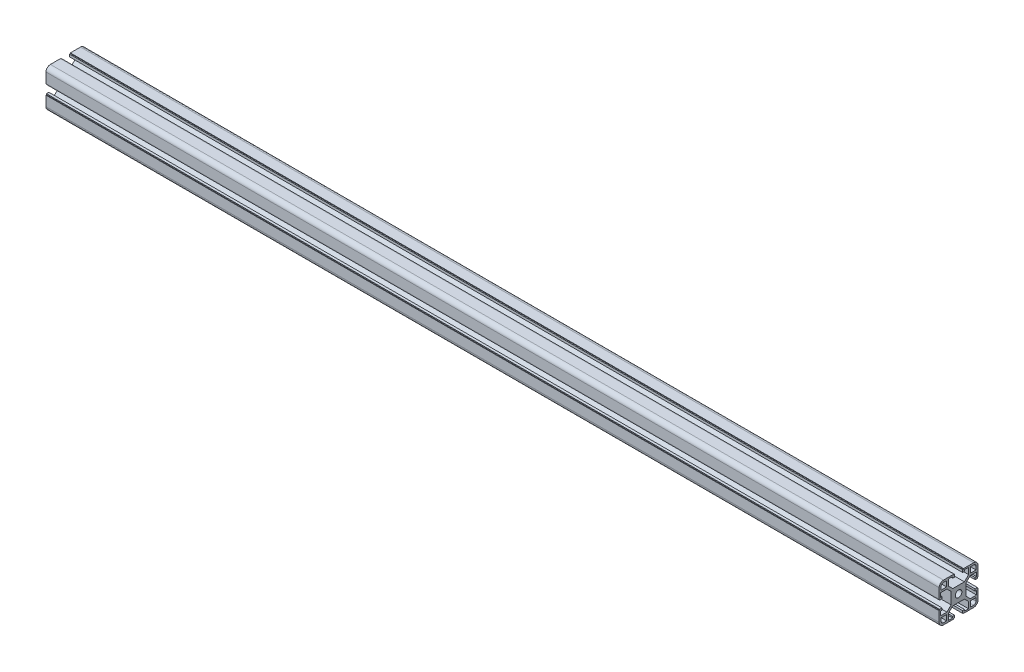
from build123d import *

# Parameters (mm, degrees)
SKETCH1_R                                = 3.4
ALUMINUM_PROFILE_40_X_40B_X_R4_5_1_DEPTH = 920


with BuildPart() as part:
    # Sketch1 → Aluminum profile 40 X 40B X R4.5(1) (new body)
    with BuildSketch(Plane.YZ):
        with BuildLine():
            Line((-5.1, 20), (-5.1, 19.5))
            Line((-5.1, 19.5), (-4.1, 19.5))
            Line((-4.1, 19.5), (-4.1, 17))
            Line((-4.1, 17), (-6.1, 17))
            Line((-6.1, 17), (-6.1, 18.5))
            Line((-6.1, 18.5), (-10.3, 18.5))
            Line((-10.3, 18.5), (-10.3, 12))
            Line((-10.3, 12), (-6, 7.7))
            Line((-6, 7.7), (6, 7.7))
            Line((6, 7.7), (10.3, 12))
            Line((10.3, 12), (10.3, 18.5))
            Line((10.3, 18.5), (6.1, 18.5))
            Line((6.1, 18.5), (6.1, 17))
            Line((6.1, 17), (4.1, 17))
            Line((4.1, 17), (4.1, 19.5))
            Line((4.1, 19.5), (5.1, 19.5))
            Line((5.1, 19.5), (5.1, 20))
            Line((5.1, 20), (15.5, 20))
            ThreePointArc((15.5, 20), (18.681980515, 18.681980515), (20, 15.5))
            Line((20, 15.5), (20, 5.1))
            Line((20, 5.1), (19.5, 5.1))
            Line((19.5, 5.1), (19.5, 4.1))
            Line((19.5, 4.1), (17, 4.1))
            Line((17, 4.1), (17, 6.1))
            Line((17, 6.1), (18.5, 6.1))
            Line((18.5, 6.1), (18.5, 10.3))
            Line((18.5, 10.3), (12, 10.3))
            Line((12, 10.3), (7.7, 6))
            Line((7.7, 6), (7.7, -6))
            Line((7.7, -6), (12, -10.3))
            Line((12, -10.3), (18.5, -10.3))
            Line((18.5, -10.3), (18.5, -6.1))
            Line((18.5, -6.1), (17, -6.1))
            Line((17, -6.1), (17, -4.1))
            Line((17, -4.1), (19.5, -4.1))
            Line((19.5, -4.1), (19.5, -5.1))
            Line((19.5, -5.1), (20, -5.1))
            Line((20, -5.1), (20, -15.5))
            ThreePointArc((20, -15.5), (18.681980515, -18.681980515), (15.5, -20))
            Line((15.5, -20), (5.1, -20))
            Line((5.1, -20), (5.1, -19.5))
            Line((5.1, -19.5), (4.1, -19.5))
            Line((4.1, -19.5), (4.1, -17))
            Line((4.1, -17), (6.1, -17))
            Line((6.1, -17), (6.1, -18.5))
            Line((6.1, -18.5), (10.3, -18.5))
            Line((10.3, -18.5), (10.3, -12))
            Line((10.3, -12), (6, -7.7))
            Line((6, -7.7), (-6, -7.7))
            Line((-6, -7.7), (-10.3, -12))
            Line((-10.3, -12), (-10.3, -18.5))
            Line((-10.3, -18.5), (-6.1, -18.5))
            Line((-6.1, -18.5), (-6.1, -17))
            Line((-6.1, -17), (-4.1, -17))
            Line((-4.1, -17), (-4.1, -19.5))
            Line((-4.1, -19.5), (-5.1, -19.5))
            Line((-5.1, -19.5), (-5.1, -20))
            Line((-5.1, -20), (-15.5, -20))
            ThreePointArc((-15.5, -20), (-18.681980515, -18.681980515), (-20, -15.5))
            Line((-20, -15.5), (-20, -5.1))
            Line((-20, -5.1), (-19.5, -5.1))
            Line((-19.5, -5.1), (-19.5, -4.1))
            Line((-19.5, -4.1), (-17, -4.1))
            Line((-17, -4.1), (-17, -6.1))
            Line((-17, -6.1), (-18.5, -6.1))
            Line((-18.5, -6.1), (-18.5, -10.3))
            Line((-18.5, -10.3), (-12, -10.3))
            Line((-12, -10.3), (-7.7, -6))
            Line((-7.7, -6), (-7.7, 6))
            Line((-7.7, 6), (-12, 10.3))
            Line((-12, 10.3), (-18.5, 10.3))
            Line((-18.5, 10.3), (-18.5, 6.1))
            Line((-18.5, 6.1), (-17, 6.1))
            Line((-17, 6.1), (-17, 4.1))
            Line((-17, 4.1), (-19.5, 4.1))
            Line((-19.5, 4.1), (-19.5, 5.1))
            Line((-19.5, 5.1), (-20, 5.1))
            Line((-20, 5.1), (-20, 15.5))
            ThreePointArc((-20, 15.5), (-18.681980515, 18.681980515), (-15.5, 20))
            Line((-15.5, 20), (-5.1, 20))
        make_face()
        Circle(SKETCH1_R, mode=Mode.SUBTRACT)
        with BuildLine():
            Line((12.3, 18), (15.5, 18))
            ThreePointArc((15.5, 18), (17.267766953, 17.267766953), (18, 15.5))
            Line((18, 15.5), (18, 12.3))
            Line((18, 12.3), (12.3, 12.3))
            Line((12.3, 12.3), (12.3, 18))
        make_face(mode=Mode.SUBTRACT)
        with BuildLine():
            Line((-15.5, 18), (-12.3, 18))
            Line((-12.3, 18), (-12.3, 12.3))
            Line((-12.3, 12.3), (-18, 12.3))
            Line((-18, 12.3), (-18, 15.5))
            ThreePointArc((-18, 15.5), (-17.267766953, 17.267766953), (-15.5, 18))
        make_face(mode=Mode.SUBTRACT)
        with BuildLine():
            Line((-18, -12.3), (-12.3, -12.3))
            Line((-12.3, -12.3), (-12.3, -18))
            Line((-12.3, -18), (-15.5, -18))
            ThreePointArc((-15.5, -18), (-17.267766953, -17.267766953), (-18, -15.5))
            Line((-18, -15.5), (-18, -12.3))
        make_face(mode=Mode.SUBTRACT)
        with BuildLine():
            Line((12.3, -12.3), (18, -12.3))
            Line((18, -12.3), (18, -15.5))
            ThreePointArc((18, -15.5), (17.267766953, -17.267766953), (15.5, -18))
            Line((15.5, -18), (12.3, -18))
            Line((12.3, -18), (12.3, -12.3))
        make_face(mode=Mode.SUBTRACT)
    extrude(amount=ALUMINUM_PROFILE_40_X_40B_X_R4_5_1_DEPTH)


solid = part.part
